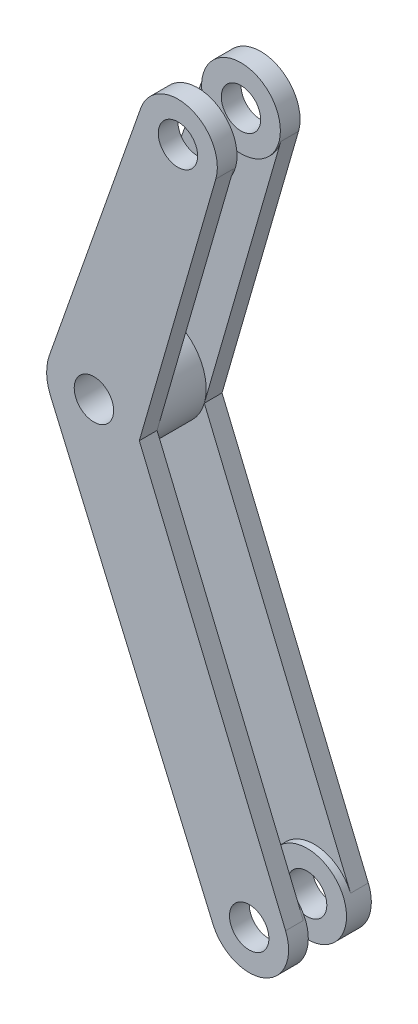
from build123d import *

# Parameters (mm, degrees)
SKETCH_1_8_R        = 100
SKETCH_1_8_R_2      = 50
SKETCH_1_8_R_3      = 120
BOSS_EXTRUDE1_DEPTH = 45
BOSS_EXTRUDE2_START = -120
SKETCH_1_3_R        = 120
SKETCH_1_3_R_2      = 50
BOSS_EXTRUDE2_DEPTH = 120
BOSS_EXTRUDE3_START = -5
SKETCH_1_4_R        = 100
SKETCH_1_4_R_2      = 50
BOSS_EXTRUDE3_DEPTH = 5
BOSS_EXTRUDE4_START = -120
SKETCH_1_6_R        = 120
SKETCH_1_6_R_2      = 50
SKETCH_1_6_R_3      = 100
BOSS_EXTRUDE4_DEPTH = 45
BOSS_EXTRUDE5_START = -120
SKETCH_1_7_R        = 50
BOSS_EXTRUDE5_DEPTH = 5
BOSS_EXTRUDE6_START = -120
SKETCH_1_8_2_R      = 50
BOSS_EXTRUDE6_DEPTH = 18


with BuildPart() as part:
    # Sketch 1_8 → Boss-Extrude1 (new body)
    # profile 1 of 5: a face of its own
    with BuildSketch(Plane.XY):
        with BuildLine():
            ThreePointArc((13620.744797989, 1922.728345575), (13494.193133773, 1855.229420726), (13430.337526965, 1983.657961365))
            Line((13430.337526965, 1983.657961365), (13198.130204679, 1323.597540284))
            ThreePointArc((13198.130204679, 1323.597540284), (13331.529491927, 1402.061952726), (13431.329633003, 1283.774313052))
            ThreePointArc((13431.329633003, 1283.774313052), (13430.146120976, 1266.962347499), (13426.618929907, 1250.482001337))
            Line((13426.618929907, 1250.482001337), (13620.744797989, 1922.728345575))
        make_face()
    # profile 2 of 5: a face of its own
    with BuildSketch(Plane.XY):
        with Locations((13524.670383902, 1950.471938671)):
            Circle(SKETCH_1_8_R)
        with Locations(Location((13524.670383902, 1950.471938671, 0), (0, 0, 180))):
            Circle(SKETCH_1_8_R_2, mode=Mode.SUBTRACT)
    # profile 3 of 5: a face of its own
    with BuildSketch(Plane.XY):
        with Locations((13311.329633003, 1283.774313052)):
            Circle(SKETCH_1_8_R_3)
        with Locations(Location((13311.329633003, 1283.774313052, 0), (0, 0, 180))):
            Circle(SKETCH_1_8_R_2, mode=Mode.SUBTRACT)
    # profile 4 of 5: a face of its own
    with BuildSketch(Plane.XY):
        with Locations((13705.595707248, 320.324645089)):
            Circle(SKETCH_1_8_R)
        with Locations(Location((13705.595707248, 320.324645089, 0), (0, 0, 180))):
            Circle(SKETCH_1_8_R_2, mode=Mode.SUBTRACT)
    # profile 5 of 5: a face of its own
    with BuildSketch(Plane.XY):
        with BuildLine():
            ThreePointArc((13426.618929907, 1250.482001337), (13318.91585359, 1164.014347884), (13201.162822108, 1236.200436006))
            Line((13201.162822108, 1236.200436006), (13613.790031502, 280.679747551))
            ThreePointArc((13613.790031502, 280.679747551), (13666.552919763, 412.387996893), (13797.912786205, 358.763647846))
            Line((13797.912786205, 358.763647846), (13426.618929907, 1250.482001337))
        make_face()
    extrude(amount=BOSS_EXTRUDE1_DEPTH)

    # 草图1<3> → Boss-Extrude2 (add)
    with BuildSketch(Plane.XY.offset(BOSS_EXTRUDE2_START)):
        with Locations(Location((13311.329633003, 1283.774313052, 0), (0, 0, 160.618277355))):
            Circle(SKETCH_1_3_R)
        with Locations(Location((13311.329633003, 1283.774313052, 0), (0, 0, 180))):
            Circle(SKETCH_1_3_R_2, mode=Mode.SUBTRACT)
    extrude(amount=BOSS_EXTRUDE2_DEPTH)

    # 草图1<4> → Boss-Extrude3 (add)
    # profile 1 of 2: a face of its own
    with BuildSketch(Plane.XY.offset(BOSS_EXTRUDE3_START)):
        with Locations(Location((13524.670383902, 1950.471938671, 0), (0, 0, 160.618277355))):
            Circle(SKETCH_1_4_R)
        with Locations(Location((13524.670383902, 1950.471938671, 0), (0, 0, 180))):
            Circle(SKETCH_1_4_R_2, mode=Mode.SUBTRACT)
    # profile 2 of 2: a face of its own
    with BuildSketch(Plane.XY.offset(BOSS_EXTRUDE3_START)):
        with Locations(Location((13705.595707248, 320.324645089, 0), (0, 0, 203.356373631))):
            Circle(SKETCH_1_4_R)
        with Locations(Location((13705.595707248, 320.324645089, 0), (0, 0, 180))):
            Circle(SKETCH_1_4_R_2, mode=Mode.SUBTRACT)
    extrude(amount=BOSS_EXTRUDE3_DEPTH)



with BuildPart() as body_2:
    # 草图1<6> → Boss-Extrude4 (new body)
    # profile 1 of 5: a face of its own
    with BuildSketch(Plane.XY.offset(BOSS_EXTRUDE4_START)):
        with BuildLine():
            ThreePointArc((13620.744797989, 1922.728345575), (13494.193133773, 1855.229420726), (13430.337526965, 1983.657961365))
            Line((13430.337526965, 1983.657961365), (13198.130204679, 1323.597540284))
            ThreePointArc((13198.130204679, 1323.597540284), (13331.529491927, 1402.061952726), (13431.329633003, 1283.774313052))
            ThreePointArc((13431.329633003, 1283.774313052), (13430.146120976, 1266.962347499), (13426.618929907, 1250.482001337))
            Line((13426.618929907, 1250.482001337), (13620.744797989, 1922.728345575))
        make_face()
    # profile 2 of 5: a face of its own
    with BuildSketch(Plane.XY.offset(BOSS_EXTRUDE4_START)):
        with BuildLine():
            ThreePointArc((13426.618929907, 1250.482001337), (13318.91585359, 1164.014347884), (13201.162822108, 1236.200436006))
            Line((13201.162822108, 1236.200436006), (13613.790031502, 280.679747551))
            ThreePointArc((13613.790031502, 280.679747551), (13666.552919763, 412.387996893), (13797.912786205, 358.763647846))
            Line((13797.912786205, 358.763647846), (13426.618929907, 1250.482001337))
        make_face()
    # profile 3 of 5: a face of its own
    with BuildSketch(Plane.XY.offset(BOSS_EXTRUDE4_START)):
        with Locations(Location((13311.329633003, 1283.774313052, 0), (0, 0, 160.618277355))):
            Circle(SKETCH_1_6_R)
        with Locations(Location((13311.329633003, 1283.774313052, 0), (0, 0, 180))):
            Circle(SKETCH_1_6_R_2, mode=Mode.SUBTRACT)
    # profile 4 of 5: a face of its own
    with BuildSketch(Plane.XY.offset(BOSS_EXTRUDE4_START)):
        with Locations(Location((13705.595707248, 320.324645089, 0), (0, 0, 203.356373631))):
            Circle(SKETCH_1_6_R_3)
        with Locations(Location((13705.595707248, 320.324645089, 0), (0, 0, 180))):
            Circle(SKETCH_1_6_R_2, mode=Mode.SUBTRACT)
    # profile 5 of 5: a face of its own
    with BuildSketch(Plane.XY.offset(BOSS_EXTRUDE4_START)):
        with Locations(Location((13524.670383902, 1950.471938671, 0), (0, 0, 160.618277355))):
            Circle(SKETCH_1_6_R_3)
        with Locations(Location((13524.670383902, 1950.471938671, 0), (0, 0, 180))):
            Circle(SKETCH_1_6_R_2, mode=Mode.SUBTRACT)
    extrude(amount=-BOSS_EXTRUDE4_DEPTH)


with BuildPart() as part_1:
    add(part.part)

    add(body_2.part)  # Boss-Extrude5 merges body 2
    # 草图1<7> → Boss-Extrude5 (add)
    with BuildSketch(Plane.XY.offset(BOSS_EXTRUDE5_START)):
        with BuildLine():
            ThreePointArc((13624.670383902, 1950.471938671), (13541.503599672, 2049.044971732), (13430.337526965, 1983.657961365))
            ThreePointArc((13430.337526965, 1983.657961365), (13494.193133773, 1855.229420726), (13620.744797989, 1922.728345575))
            ThreePointArc((13620.744797989, 1922.728345575), (13623.684123879, 1936.461967377), (13624.670383902, 1950.471938671))
        make_face()
        with Locations(Location((13524.670383902, 1950.471938671, 0), (0, 0, 180))):
            Circle(SKETCH_1_7_R, mode=Mode.SUBTRACT)
    extrude(amount=BOSS_EXTRUDE5_DEPTH)

    # Sketch 1_8 2 → Boss-Extrude6 (add)
    with BuildSketch(Plane.XY.offset(BOSS_EXTRUDE6_START)):
        with BuildLine():
            ThreePointArc((13797.912786205, 358.763647846), (13666.552919763, 412.387996893), (13613.790031502, 280.679747551))
            ThreePointArc((13613.790031502, 280.679747551), (13725.837155139, 222.39465077), (13805.595707248, 320.324645089))
            ThreePointArc((13805.595707248, 320.324645089), (13803.656167924, 339.924289274), (13797.912786205, 358.763647846))
        make_face()
        with Locations(Location((13705.595707248, 320.324645089, 0), (0, 0, 180))):
            Circle(SKETCH_1_8_2_R, mode=Mode.SUBTRACT)
    extrude(amount=BOSS_EXTRUDE6_DEPTH)


solid = part_1.part
